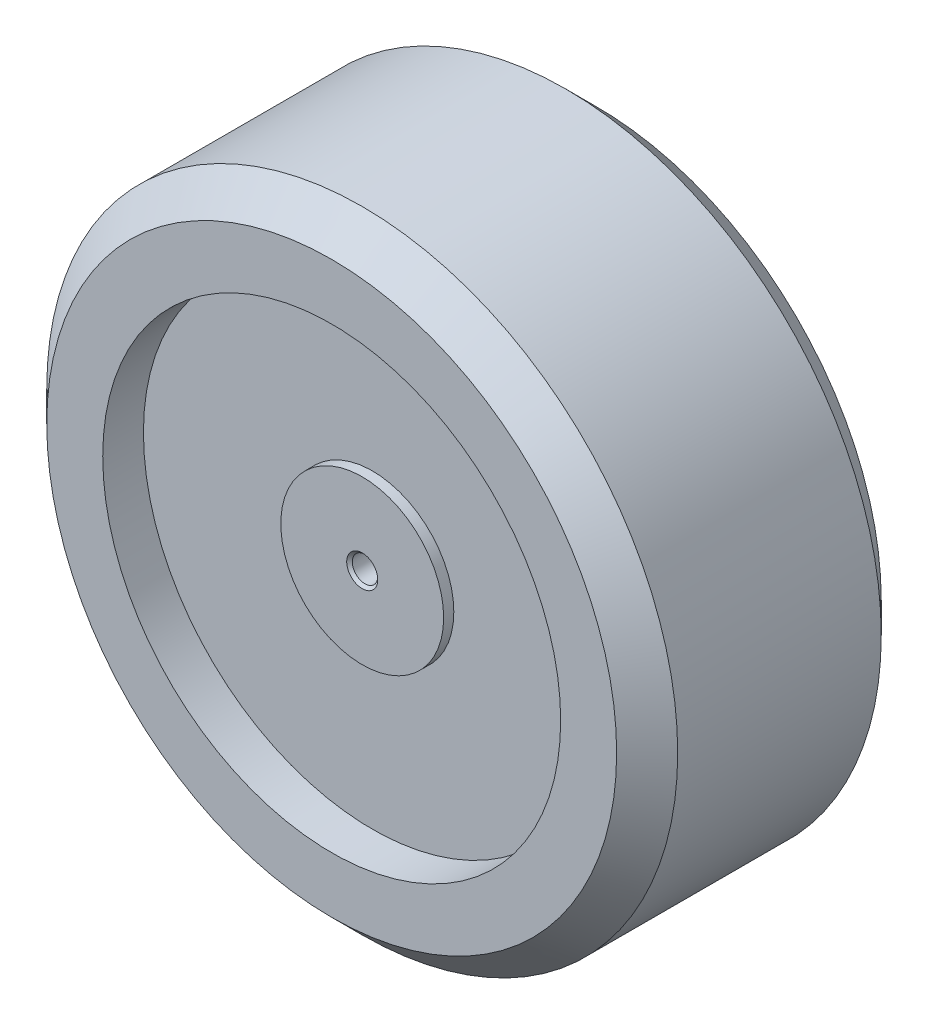
from build123d import *

# Parameters (mm, degrees)
SKETCH1_R                   = 31
BOSS_EXTRUDE1_DEPTH         = 26
SKETCH2_R                   = 22.5
CUT_EXTRUDE1_DEPTH          = 11
CUT_EXTRUDE2_DEPTH          = 3.1
CUT_EXTRUDE3_START          = -4
SKETCH4_R                   = 22.5
SKETCH4_R_2                 = 8
CUT_EXTRUDE3_DEPTH          = 4
CUT_EXTRUDE4_START          = -3
SKETCH5_R                   = 8
CUT_EXTRUDE4_DEPTH          = 3
M3_TAPPED_HOLE1_D           = 2.5
M3_TAPPED_HOLE1_CSINK_D     = 3.05
M3_TAPPED_HOLE1_CSINK_ANGLE = 90
CHAMFER1_SIZE               = 3


with BuildPart() as part:
    # Sketch1 → Boss-Extrude1 (new body)
    with BuildSketch(Plane.XY):
        with Locations(Location((0, 0, 0), (0, 0, 180))):
            Circle(SKETCH1_R)
    extrude(amount=BOSS_EXTRUDE1_DEPTH)

    # Sketch2 → Cut-Extrude1 (cut)
    with BuildSketch(Plane(origin=(0, 0, 0), x_dir=(-1, 0, 0), z_dir=(0, 0, -1))):
        Circle(SKETCH2_R)
    extrude(amount=-CUT_EXTRUDE1_DEPTH, mode=Mode.SUBTRACT)

    # Sketch3 → Cut-Extrude2 (cut)
    with BuildSketch(Plane(origin=(0, 0, 11), x_dir=(-1, 0, 0), z_dir=(0, 0, -1))):
        Polygon((0, 6.92820323), (-6, 3.464101615), (-6, -3.464101615), (0, -6.92820323), (6, -3.464101615), (6, 3.464101615), align=None)
    extrude(amount=-CUT_EXTRUDE2_DEPTH, mode=Mode.SUBTRACT)

    # Sketch4 → Cut-Extrude3 (cut)
    with BuildSketch(Plane.XY.offset(26).offset(CUT_EXTRUDE3_START)):
        with Locations(Location((0, 0, 0), (0, 0, 180))):
            Circle(SKETCH4_R)
        Circle(SKETCH4_R_2, mode=Mode.SUBTRACT)
    extrude(amount=CUT_EXTRUDE3_DEPTH, mode=Mode.SUBTRACT)

    # Sketch5 → Cut-Extrude4 (cut)
    with BuildSketch(Plane.XY.offset(26).offset(CUT_EXTRUDE4_START)):
        Circle(SKETCH5_R)
    extrude(amount=CUT_EXTRUDE4_DEPTH, mode=Mode.SUBTRACT)

    # M3 Tapped Hole1 (through all)
    with Locations(Plane.XY.offset(23)):
        with Locations((0, 0)):
            CounterSinkHole(M3_TAPPED_HOLE1_D / 2, M3_TAPPED_HOLE1_CSINK_D / 2, counter_sink_angle=M3_TAPPED_HOLE1_CSINK_ANGLE)

    # Chamfer1
    chamfer1_edges = [part.edges().sort_by_distance(p)[0] for p in [
        (31, 0, 0),
        (31, 0, 26),
    ]]
    chamfer(chamfer1_edges, length=CHAMFER1_SIZE)


solid = part.part
